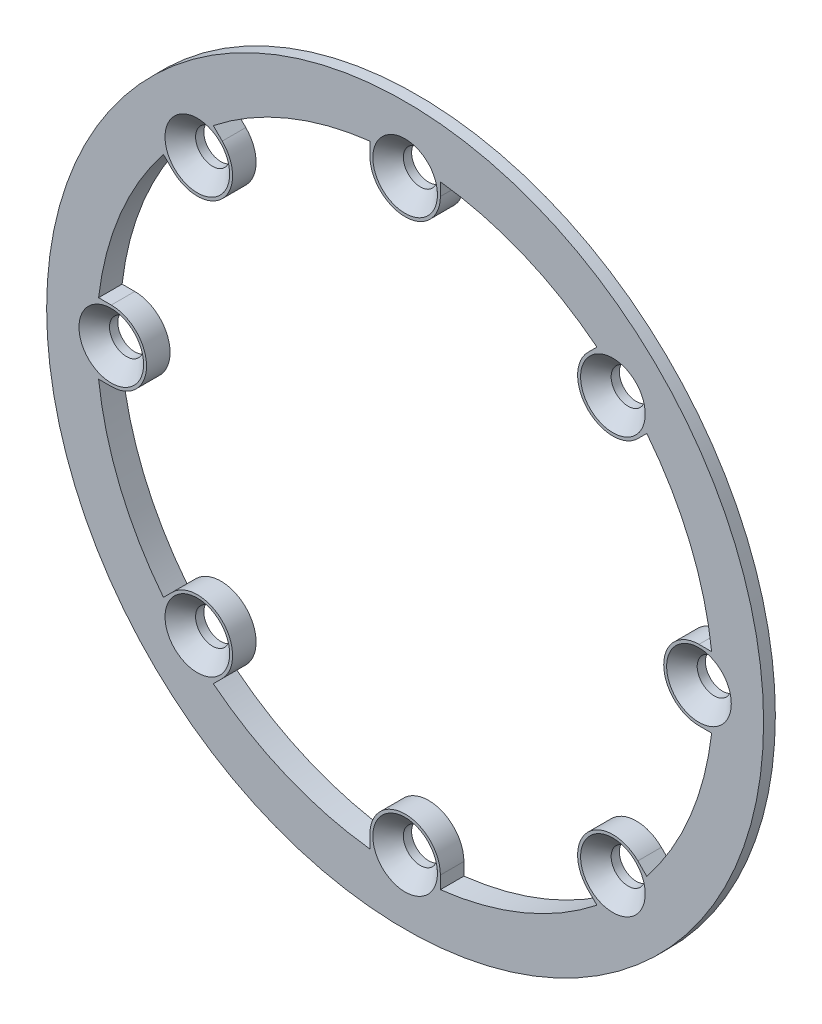
from build123d import *

# Parameters (mm, degrees)
SKETCH1_R           = 30.5
SKETCH1_R_2         = 26.25
BOSS_EXTRUDE1_DEPTH = 1
CHAMFER1_SIZE       = 1.5
CHAMFER1_SIZE2      = 1
BOSS_EXTRUDE2_START = -2
BOSS_EXTRUDE2_DEPTH = 2
CIRPATTERN2_COUNT   = 8


with BuildPart() as part:
    # Sketch1 → Boss-Extrude1 (new, symmetric)
    with BuildSketch(Plane.XY):
        Circle(SKETCH1_R)
        Circle(SKETCH1_R_2, mode=Mode.SUBTRACT)
    extrude(amount=BOSS_EXTRUDE1_DEPTH, both=True)

    # Chamfer1
    chamfer1_edges = [part.edges().sort_by_distance(p)[0] for p in [
        (-30.5, 0, -1),
    ]]
    chamfer1_side = [part.faces().sort_by_distance(p)[0] for p in [
        (-29.637329727, 0, -1),
    ]]
    chamfer(chamfer1_edges, length=CHAMFER1_SIZE, length2=CHAMFER1_SIZE2, reference=chamfer1_side[0])

    # Sketch4 → Boss-Extrude2 (add)
    with BuildSketch(Plane.XY.offset(1).offset(BOSS_EXTRUDE2_START)):
        with BuildLine():
            Line((-3, 25), (-3, 26.078007976))
            ThreePointArc((-3, 26.078007976), (0, 26.25), (3, 26.078007976))
            Line((3, 26.078007976), (3, 25))
            ThreePointArc((3, 25), (0, 22), (-3, 25))
        make_face()
    boss_extrude2 = extrude(amount=BOSS_EXTRUDE2_DEPTH)

    # Sketch5 → CSK for M2.5 Countersunk Flat Head Screw2 (revolve, cut)
    with BuildSketch(Plane(origin=(0, 25, 1), x_dir=(0, -1, 0), z_dir=(1, 0, 0))):
        Polygon((0, 0), (0, 2), (1.45, 2), (1.45, 1.3), (2.75, 0), align=None)
    csk_for_m2_5_countersunk_flat_head_screw = revolve(axis=Axis((0, 25, 7.35), (0, 0, -1)), mode=Mode.SUBTRACT)

    # CirPattern2: Boss-Extrude2, CSK for M2.5 Countersunk Flat Head Screw2 ×8 about axis
    cirpattern2_axis = Axis((0, 0, 0), (0, 0, 1))
    add([boss_extrude2.rotate(cirpattern2_axis, i * 360 / CIRPATTERN2_COUNT) for i in range(1, CIRPATTERN2_COUNT)])
    add([csk_for_m2_5_countersunk_flat_head_screw.rotate(cirpattern2_axis, i * 360 / CIRPATTERN2_COUNT) for i in range(1, CIRPATTERN2_COUNT)], mode=Mode.SUBTRACT)


solid = part.part
